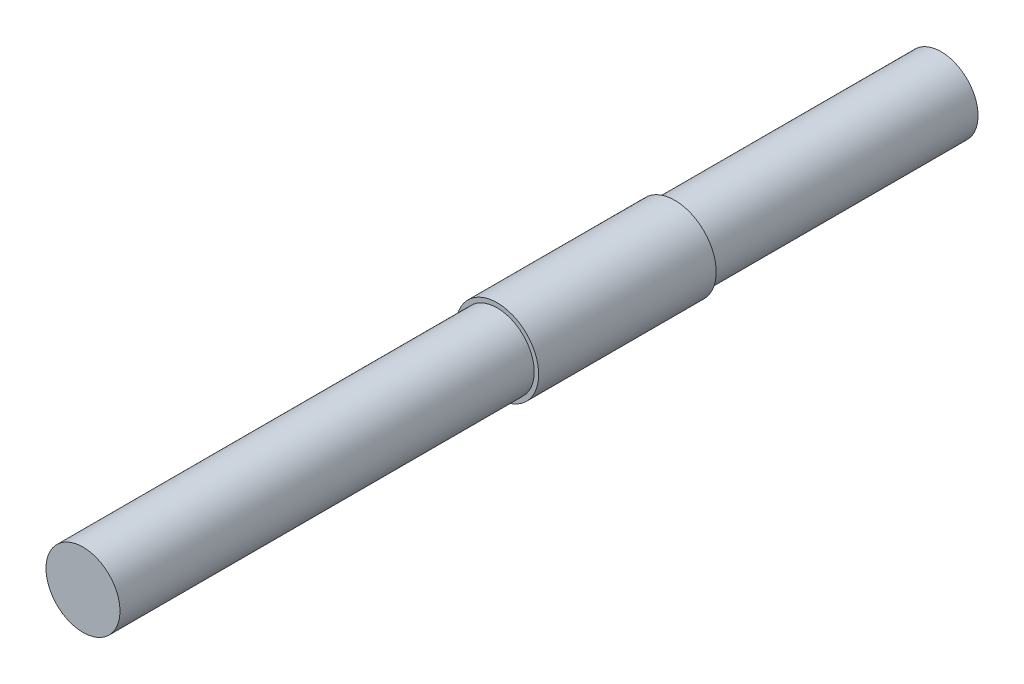
from build123d import *


with BuildPart() as part:
    # Sketch1 → Revolve1 (revolve)
    with BuildSketch(Plane.XZ.offset(-889.976481234), mode=Mode.PRIVATE) as revolve1_sk:
        Polygon((533.730642584, -100.892981355), (521.230642584, -100.892981355), (521.230642584, -390.892981355), (533.730642584, -390.892981355), (533.730642584, -300.892981355), (535.230642584, -300.892981355), (535.230642584, -240.892981355), (533.730642584, -240.892981355), align=None)
    revolve(revolve1_sk.sketch.rotate(Axis((521.230642584, 889.976481234, -100.892981355), (0, 0, -1)), 180), axis=Axis((521.230642584, 889.976481234, -100.892981355), (0, 0, -1)))


solid = part.part
